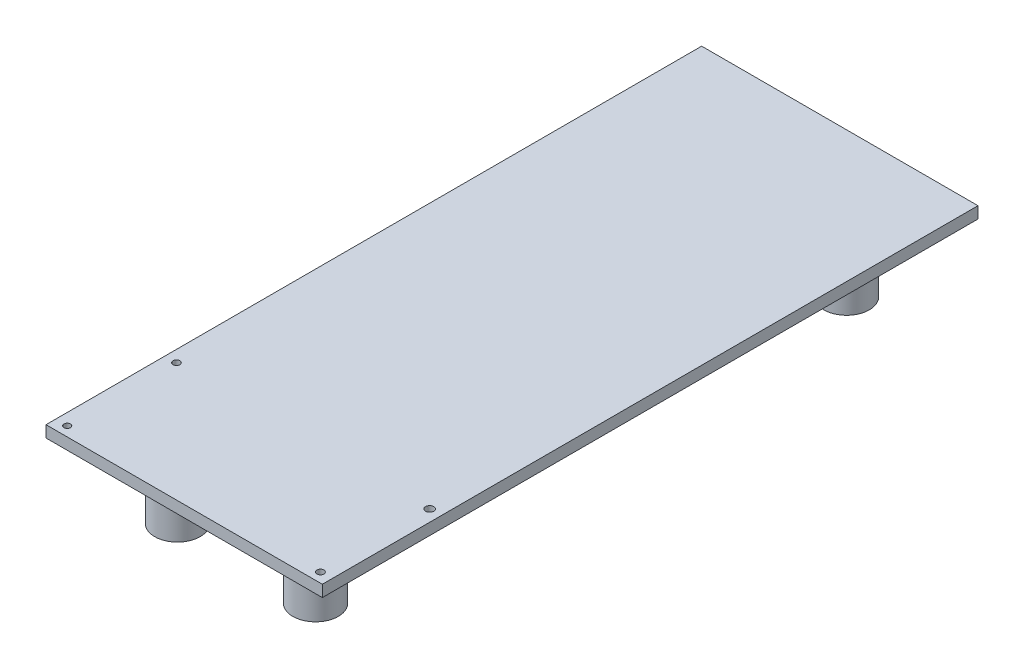
SolidWorks part; units mm, degrees
ref_plane "Front Plane" through (0, 0, 0) normal (0, 0, 1) x (1, 0, 0)
ref_plane "Top Plane" through (0, 0, 0) normal (0, 1, 0) x (1, 0, 0)
ref_plane "Right Plane" through (0, 0, 0) normal (1, 0, 0) x (0, 0, -1)
sketch "Sketch1" plane through (0, 0, 0) normal (0, 1, 0) x (1, 0, 0)
  line L0 (-180.8023, 530.1746) -> (-230.8023, 530.1746) construction
  line L13 (204.1977, -490.0734) -> (-225.8023, -490.0734)
  line L16 (-225.8023, -490.0734) -> (-225.8023, -290.0734)
  line L19 (204.1977, 530.1746) -> (-225.8023, 530.1746)
  line L20 (-225.8023, -290.0734) -> (-225.8023, 530.1746)
  line L21 (204.1977, -490.0734) -> (204.1977, 530.1746)
  circle A0 centre (186.1977, -475.0734) radius 5.5
  circle A1 centre (186.1977, -305.0734) radius 6.3605
  circle A2 centre (-207.8023, -305.0734) radius 5.3512
  circle A3 centre (-207.8023, -475.0734) radius 5.0792
extrude "Boss-Extrude1" add sketch "Sketch1" along normal blind 18
sketch "Sketch2" plane through (0, 0, 0) normal (0, -1, 0) x (1, 0, 0)
  circle A0 centre (96.6655, 393.0732) radius 35.3897
  circle A1 centre (-118.2701, 393.0732) radius 35.3897
  circle A2 centre (-118.2701, -433.1744) radius 35.3897
  circle A3 centre (96.6655, -433.1744) radius 35.3897
extrude "Boss-Extrude2" add sketch "Sketch2" along normal blind 110
